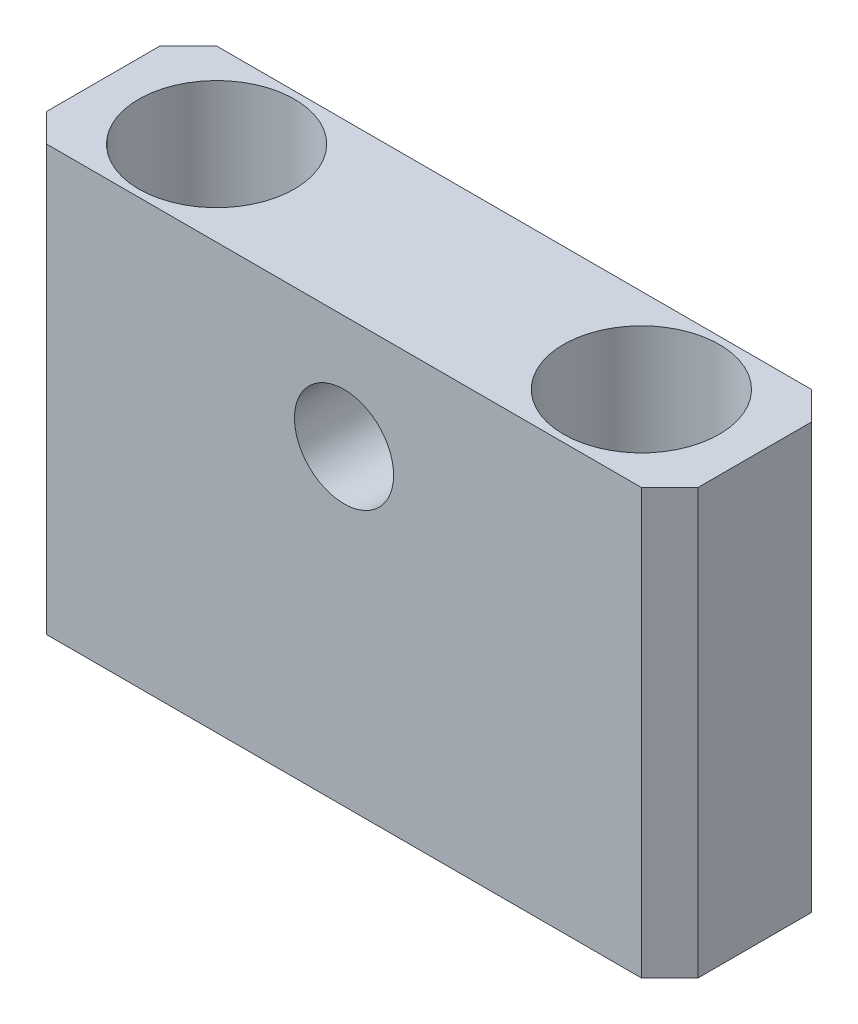
SolidWorks part; units mm, degrees
ref_plane "前视基准面" through (0, 0, 0) normal (0, 0, 1) x (1, 0, 0)
ref_plane "上视基准面" through (0, 0, 0) normal (0, 1, 0) x (1, 0, 0)
ref_plane "右视基准面" through (0, 0, 0) normal (1, 0, 0) x (0, 0, -1)
sketch "草图1" plane through (0, 0, 0) normal (0, 0, 1) x (1, 0, 0)
  line L1 (0, 0) -> (46, 0)
  line L2 (0, 0) -> (0, 30)
  line L3 (0, 30) -> (46, 30)
  line L4 (46, 0) -> (46, 30)
  dimension "D1" = 30
  dimension "D2" = 46
extrude "凸台-拉伸1" add sketch "草图1" along normal blind 12
hole_wizard "Ø7.0 (7) 直径孔1" positions "草图3" profile "草图4" hole size "Ø7.0" standard "GB" end condition through all
sketch "草图3" plane through (0, 0, 12) normal (0, 0, 1) x (1, 0, 0)
  line L0 (23, 0) -> (23, 31.6158) construction
  line L1 (0, 0) -> (46, 0) construction
  point P0 (23, 22)
  dimension "D1" = 22
sketch "草图4" plane through (23, 22, 12) normal (1, 0, 0) x (0, -1, 0)
  line L0 (0, 0) -> (0, 12)
  line L1 (0, 12) -> (3.5, 12)
  line L2 (3.5, 12) -> (3.5, 0)
  line L5 (3.5, 0) -> (0, 0)
  line L11 (0, -6.35) -> (0, 107.95) construction
  dimension "通孔孔直径" = 7
  dimension "通孔孔深度" = 12
hole_wizard "M6 六角凹头螺钉的柱形沉头孔1" positions "草图6" profile "草图5" counterbore size "M6" standard "ISO" end condition through all
sketch "草图6" plane through (0, 30, 0) normal (0, 1, 0) x (1, 0, 0)
  line L0 (0, -6) -> (46, -6) construction
  line L1 (0, -12) -> (0, 0) construction
  line L2 (46, -12) -> (46, 0) construction
  line L4 (23, 0) -> (23, -12) construction
  line L5 (46, 0) -> (0, 0) construction
  line L6 (46, -12) -> (0, -12) construction
  point P0 (8, -6)
  point P2 (38, -6)
  dimension "D1" = 30
sketch "草图5" plane through (8, 30, 6) normal (1, 0, 0) x (0, 0, 1)
  line L0 (0, 0) -> (0, 30)
  line L1 (0, 30) -> (3.2, 30)
  line L3 (3.2, 30) -> (3.2, 6.4)
  line L4 (3.2, 6.4) -> (5.5, 6.4)
  line L5 (5.5, 6.4) -> (5.5, 0)
  line L7 (5.5, 0) -> (0, 0)
  line L11 (0, -6.35) -> (0, 107.95) construction
  dimension "通孔孔直径" = 6.4
  dimension "通孔孔深度" = 30
  dimension "柱形沉头孔直径" = 11
  dimension "柱形沉头孔深度" = 6.4
sketch "草图7" plane through (0, 23.6, 0) normal (0, 1, 0) x (1, 0, 0)
  circle A0 centre (8, -6) radius 5.5 construction
  circle A1 centre (38, -6) radius 5.5 construction
  circle A2 centre (8, -6) radius 5.5
  circle A3 centre (38, -6) radius 5.5
extrude "切除-拉伸1" cut sketch "草图7" against normal blind 10
chamfer "倒角1" distance 2 angle 45 4 edges at (0, 15, 12) (0, 15, 0) (46, 15, 12) (46, 15, 0)
